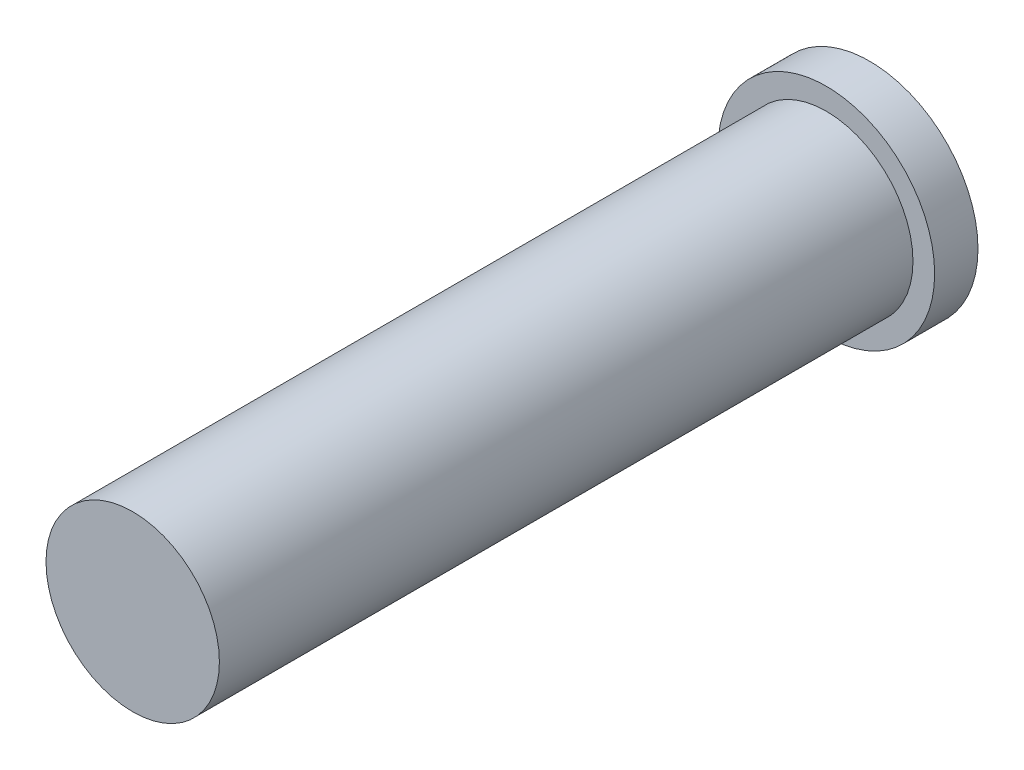
SolidWorks part; units mm, degrees
ref_plane "前视基准面" through (0, 0, 0) normal (0, 0, 1) x (1, 0, 0)
ref_plane "上视基准面" through (0, 0, 0) normal (0, 1, 0) x (1, 0, 0)
ref_plane "右视基准面" through (0, 0, 0) normal (1, 0, 0) x (0, 0, -1)
sketch "草图1" plane through (0, 0, 0) normal (0, 0, 1) x (1, 0, 0)
  circle A0 centre (0, 0) radius 2.5
  dimension "D1" = 5
extrude "凸台-拉伸1" add sketch "草图1" along normal blind 1
sketch "草图2" plane through (0, 0, 1) normal (0, 0, 1) x (1, 0, 0)
  circle A0 centre (0, 0) radius 2
  dimension "D1" = 4
extrude "凸台-拉伸2" add sketch "草图2" along normal blind 16
